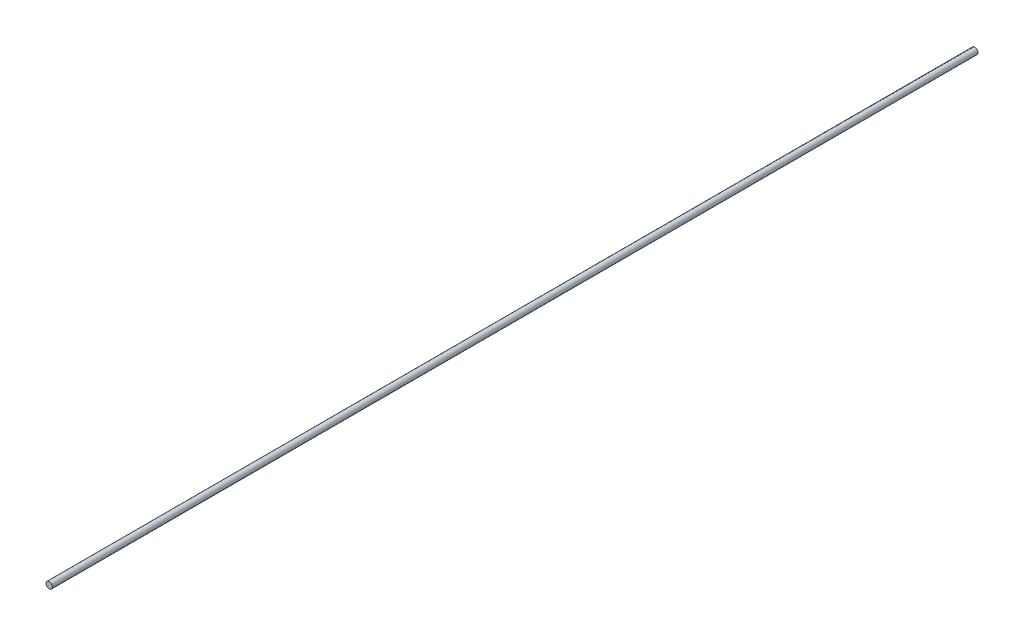
from build123d import *

# Parameters (mm, degrees)
SKETCH1_R           = 3
BOSS_EXTRUDE1_DEPTH = 875


with BuildPart() as part:
    # Sketch1 → Boss-Extrude1 (new body)
    with BuildSketch(Plane.XY):
        Circle(SKETCH1_R)
    extrude(amount=BOSS_EXTRUDE1_DEPTH)


solid = part.part
